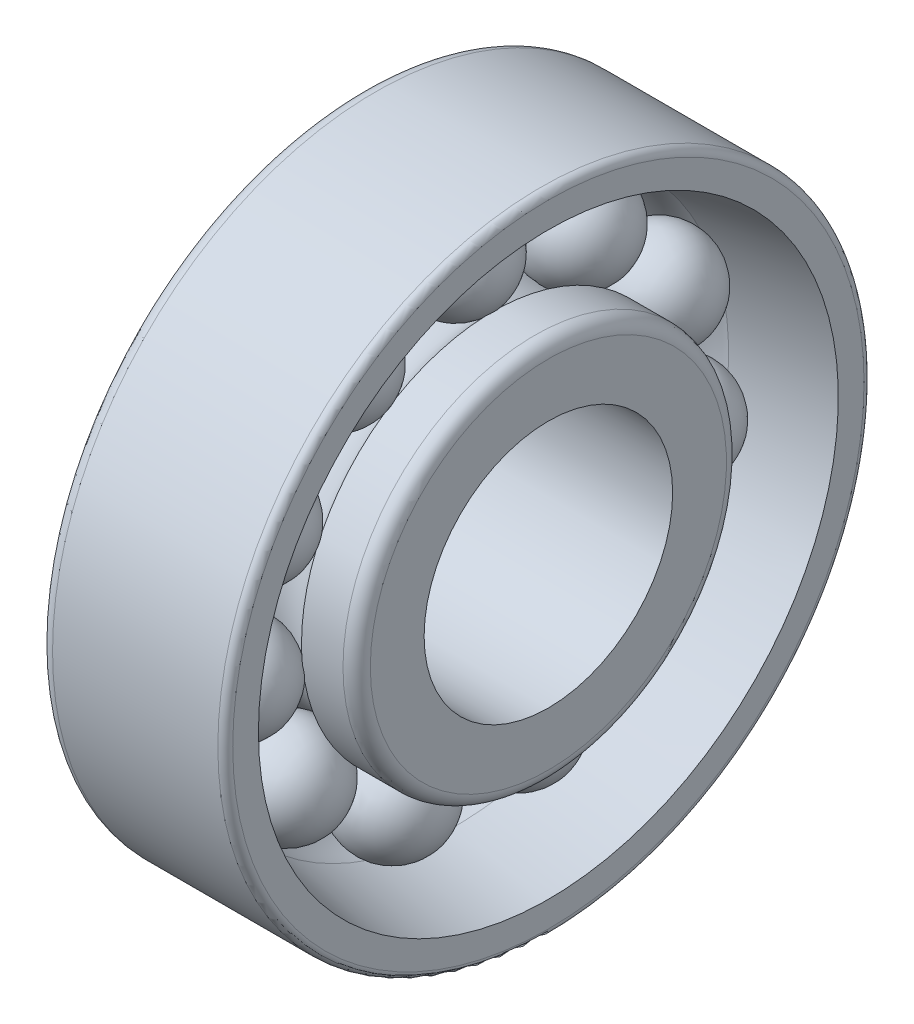
SolidWorks part; units mm, degrees
ref_plane "Front" through (0, 0, 0) normal (0, 0, 1) x (1, 0, 0)
ref_plane "Top" through (0, 0, 0) normal (0, 1, 0) x (1, 0, 0)
ref_plane "Right" through (0, 0, 0) normal (1, 0, 0) x (0, 0, -1)
sketch "Dimension Sketch" plane through (0, 0, 0) normal (0, 0, 1) x (1, 0, 0)
  line L0 (-3.205, -4.1476) -> (48.795, -4.1476)
  point P2 (16.795, -4.1476)
  point P3 (1.795, -4.1476)
  point P4 (0.7517, -4.1476)
  point P7 (48.195, -4.1476)
  point P8 (47.695, -4.1476)
sketch "Sketch1" plane through (0, 0, 0) normal (0, 0, 1) x (1, 0, 0)
  line L0 (0, 0) -> (106.1418, 0) construction
  line L1 (0, 0) -> (0, 122.9209) construction
  line L2 (0, 26) -> (15, 26)
  line L3 (0, 10) -> (15, 10)
  line L4 (0, 26) -> (0, 10)
  line L5 (15, 26) -> (15, 15.4288)
  line L6 (15, 10) -> (15, 15.4288)
  line L7 (15, 15.4288) -> (0, 15.4288)
  line L9 (0, 18) -> (95.9613, 18) construction
  line L10 (7.5, 0) -> (7.5, 122.9209) construction
  line L11 (7.5, 22) -> (14, 22)
  line L12 (4.4358, 20.5712) -> (0, 20.5712)
  line L13 (14, 22) -> (14, 23.3333)
  line L14 (14, 23.3333) -> (15, 23.3333)
  line L15 (7.5, 18) -> (4.4358, 20.5712) construction
  circle A0 centre (7.5, 18) radius 4
sketch "Sketch2" plane through (0, 0, 0) normal (0, 0, 1) x (1, 0, 0)
  line L0 (14, 22) -> (14, 23.3333) construction
  line L1 (14, 23.3333) -> (15, 23.3333) construction
  line L2 (0, 26) -> (15, 26) construction
  line L3 (7.5, 22) -> (14, 22) construction
  line L4 (4.4358, 20.5712) -> (0, 20.5712) construction
  line L5 (0, 0) -> (106.1418, 0) construction
  line L6 (14, 22) -> (14, 23.3333) construction
  line L7 (14, 23.3333) -> (15, 23.3333) construction
  line L8 (0, 26) -> (15, 26)
  line L9 (7.5, 22) -> (14, 22) construction
  line L10 (4.4358, 20.5712) -> (0, 20.5712)
  line L11 (0, 0) -> (106.1418, 0) construction
  line L12 (15, 26) -> (15, 15.4288) construction
  line L13 (0, 26) -> (0, 10) construction
  line L14 (15, 26) -> (15, 23.3333)
  line L15 (0, 26) -> (0, 20.5712)
  line L16 (15, 23.3333) -> (7.5, 22)
  circle A0 centre (7.5, 18) radius 4 construction
  arc A1 (7.5, 22) -> (4.4358, 20.5712) centre (7.5, 18) ccw
revolve "Base-Revolve" add sketch "Sketch2" angle 360 about L11
sketch "Sketch3" plane through (0, 0, 0) normal (0, 0, 1) x (1, 0, 0)
  line L0 (0, 18) -> (95.9613, 18) construction
  line L1 (0, 18) -> (95.9613, 18) construction
  line L2 (11.55, 18) -> (3.45, 18)
  arc A0 (11.55, 18) -> (3.45, 18) centre (7.5, 18) ccw
  circle A1 centre (7.5, 18) radius 4
  arc A2 (11.5, 18) -> (3.5, 18) centre (7.5, 18) ccw construction
  dimension "D1" = 0
  dimension "D2" = 0.05
revolve "Boss-Revolve1" add sketch "Sketch3" angle 360 about L1
sketch "Sketch4" plane through (0, 0, 0) normal (0, 0, 1) x (1, 0, 0)
  line L0 (15, 10) -> (15, 15.4288) construction
  line L1 (0, 26) -> (0, 10) construction
  line L2 (0, 10) -> (15, 10) construction
  line L3 (15, 15.4288) -> (0, 15.4288) construction
  line L4 (15, 10) -> (15, 15.4288)
  line L5 (4.4358, 15.4288) -> (0, 15.4288)
  line L6 (0, 10) -> (15, 10)
  line L7 (15, 15.4288) -> (10.5642, 15.4288)
  line L8 (0, 0) -> (106.1418, 0) construction
  line L9 (0, 0) -> (106.1418, 0) construction
  line L11 (0, 15.4288) -> (0, 10)
  circle A0 centre (7.5, 18) radius 4 construction
  arc A1 (4.4358, 15.4288) -> (10.5642, 15.4288) centre (7.5, 18) ccw
revolve "Boss-Revolve2" add sketch "Sketch4" angle 360 about L9
fillet "Fillet1" radius 0.6 1 edges at (15, 0, 26)
fillet "Fillet2" radius 1.1 2 edges at (15, 0, 15.4288) (0, 0, 26)
pattern_circular "CirPattern2" count 11 over 360 about axis through (0, 0, 0) along (1, 0, 0) of "Boss-Revolve1"
equation "\"D5@Sketch1\" = \"DD@Dimension Sketch\""
equation "\"D6@Sketch1\" = \"B@Dimension Sketch\""
equation "\"D1@Fillet2\" = \"r@Dimension Sketch\""
equation "\"D1@Fillet1\" = \"r1@Dimension Sketch\""
equation "\"D4@Sketch1\" = \"d@Dimension Sketch\""
equation "\"D1@CirPattern2\" =3.14* (  \"DD@Dimension Sketch\" + \"d@Dimension Sketch\" )  / 2/ (  ( \"DD@Dimension Sketch\" - \"d@Dimension Sketch\" )  / 3 ) "
equation "\"D1@Sketch1\" = \"D6@Sketch1\""
equation "\"D2@Sketch1\" = \"D1@Sketch1\" / 2"
equation "\"D9@Sketch1\" =   ( \"D5@Sketch1\" - \"D4@Sketch1\" )  /6"
equation "\"D8@Sketch1\" =  ( \"D5@Sketch1\" - \"D4@Sketch1\" )  / 8"
